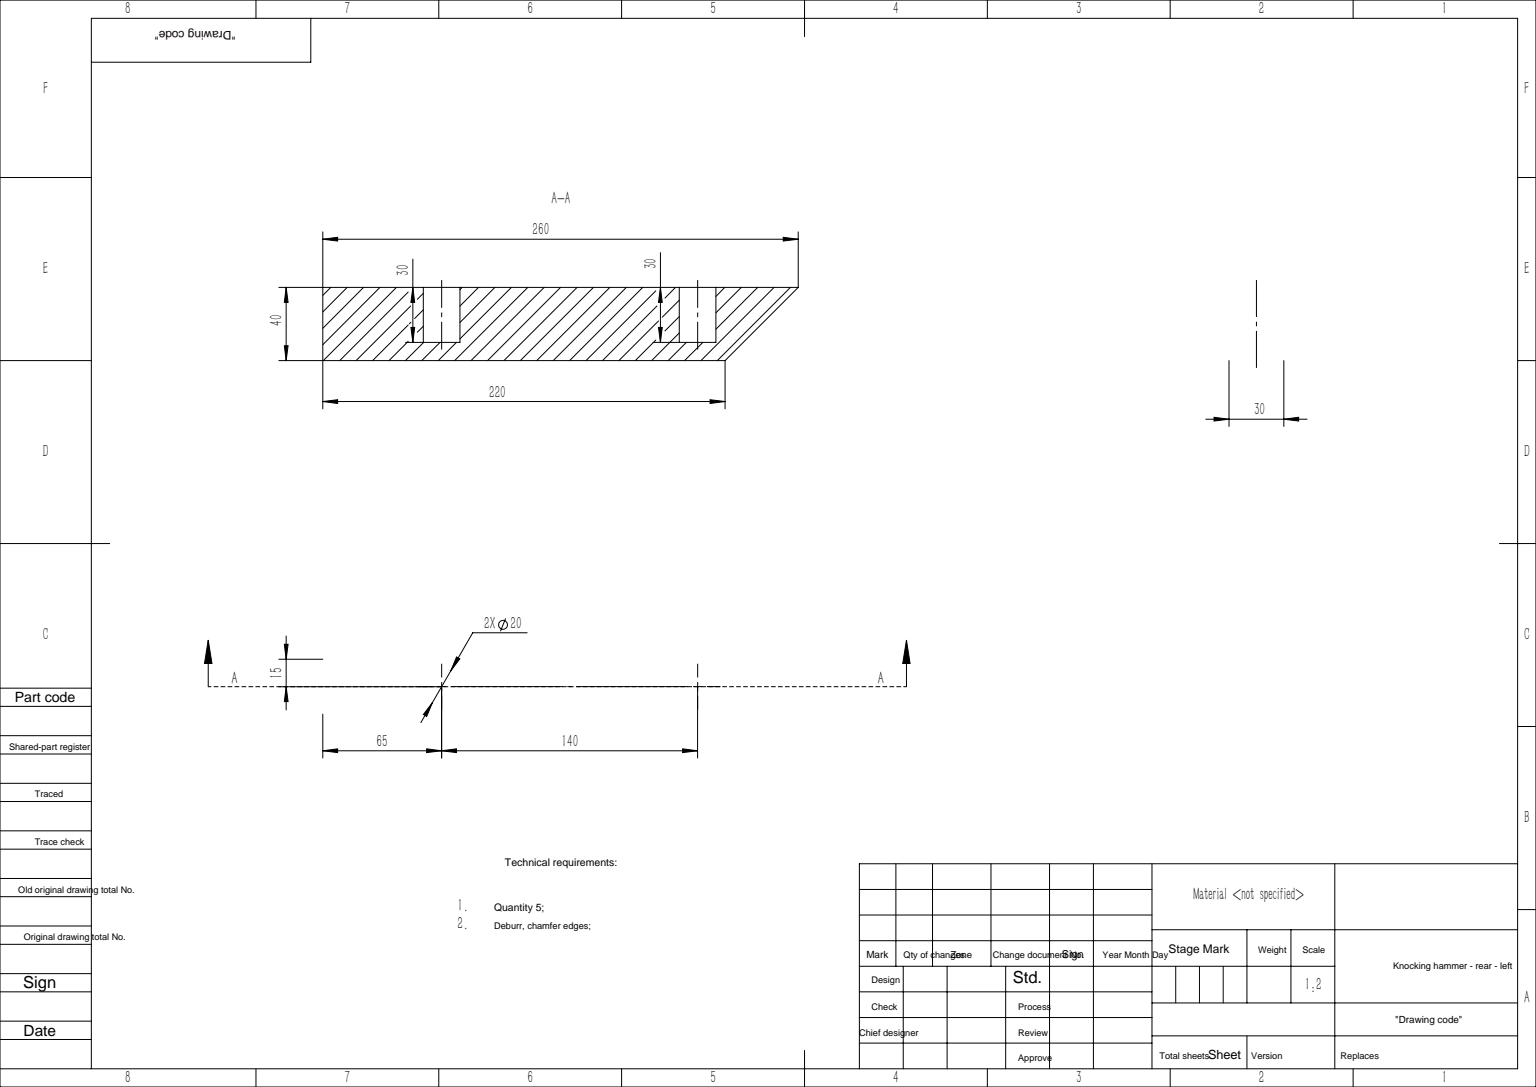
from build123d import *

# Parameters (mm, degrees)
SKETCH_1_W          = 270
SKETCH_1_H          = 30
EXTRUDE_1_DEPTH     = 40
SKETCH_2_R          = 10
CUT_EXTRUDE_2_DEPTH = 30
SKETCH_5_W          = 30
SKETCH_5_H          = 40
CUT_EXTRUDE_4_DEPTH = 10
CUT_EXTRUDE_5_DEPTH = 144.961800489


with BuildPart() as part:
    # 草图1 → 凸台-拉伸1 (new body)
    with BuildSketch(Plane(origin=(0, 0, 0), x_dir=(1, 0, 0), z_dir=(0, 1, 0))):
        Rectangle(SKETCH_1_W, SKETCH_1_H)
    extrude(amount=EXTRUDE_1_DEPTH)

    # 草图2 → 切除-拉伸2 (cut)
    with BuildSketch(Plane(origin=(0, 40, 0), x_dir=(1, 0, 0), z_dir=(0, 1, 0))):
        with Locations(Location((70, 0, 0), (0, 0, 270))):
            Circle(SKETCH_2_R)
        with Locations(Location((-70, 0, 0), (0, 0, 90))):
            Circle(SKETCH_2_R)
    extrude(amount=-CUT_EXTRUDE_2_DEPTH, mode=Mode.SUBTRACT)

    # 草图5 → 切除-拉伸4 (cut)
    with BuildSketch(Plane(origin=(135, 0, 0), x_dir=(0, 0, -1), z_dir=(1, 0, 0))):
        with Locations((0, 20)):
            Rectangle(SKETCH_5_W, SKETCH_5_H)
    extrude(amount=-CUT_EXTRUDE_4_DEPTH, mode=Mode.SUBTRACT)

    # 草图6 → 切除-拉伸5 (cut, through all)
    with BuildSketch(Plane.XY.offset(15)):
        Polygon((125, 40), (85, 0), (125, 0), align=None)
    extrude(amount=-CUT_EXTRUDE_5_DEPTH, mode=Mode.SUBTRACT)


solid = part.part
